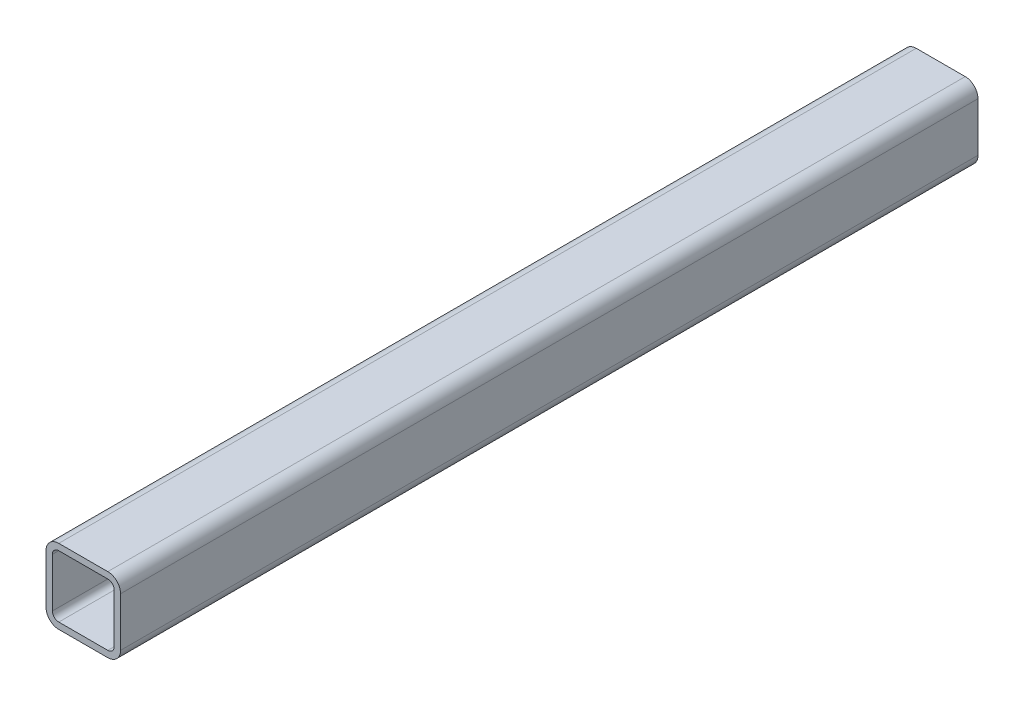
SolidWorks part; units mm, degrees
material "方管70×6/不锈钢304"
ref_plane "Front Plane" through (0, 0, 0) normal (0, 0, 1) x (1, 0, 0)
ref_plane "Top Plane" through (0, 0, 0) normal (0, 1, 0) x (1, 0, 0)
ref_plane "Right Plane" through (0, 0, 0) normal (1, 0, 0) x (0, 0, -1)
sketch "Sketch1" plane through (0, 0, 0) normal (0, 0, 1) x (1, 0, 0)
  line L1 (12, 0) -> (58, 0)
  line L2 (0, 12) -> (0, 58)
  line L3 (12, 70) -> (58, 70)
  line L4 (70, 12) -> (70, 58)
  line L5 (12, 6) -> (58, 6)
  line L6 (6, 12) -> (6, 58)
  line L7 (12, 64) -> (58, 64)
  line L8 (64, 12) -> (64, 58)
  arc A0 (12, 6) -> (6, 12) centre (12, 12) cw
  arc A1 (58, 6) -> (64, 12) centre (58, 12) ccw
  arc A2 (58, 64) -> (64, 58) centre (58, 58) cw
  arc A3 (6, 58) -> (12, 64) centre (12, 58) cw
  arc A4 (12, 0) -> (0, 12) centre (12, 12) cw
  arc A5 (58, 0) -> (70, 12) centre (58, 12) ccw
  arc A6 (58, 70) -> (70, 58) centre (58, 58) cw
  arc A7 (0, 58) -> (12, 70) centre (12, 58) cw
  point P19 (0, 0)
  point P22 (70, 0)
  point P27 (0, 70)
  dimension "D7" = 6
  dimension "D8" = 12
  dimension "D1" = 70
  dimension "D2" = 70
  dimension "D3" = 6
  dimension "D4" = 6
  dimension "D5" = 6
  dimension "D6" = 6
extrude "Boss-Extrude1" add sketch "Sketch1" along normal blind 805
